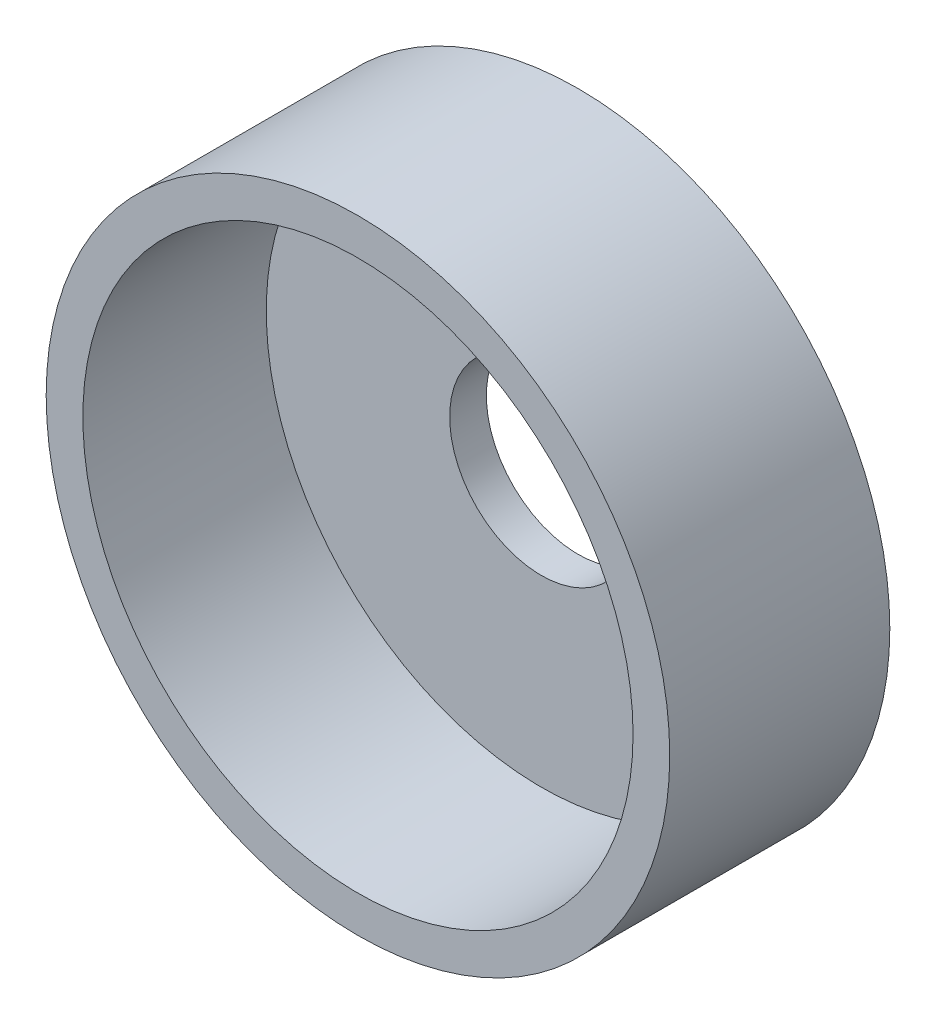
SolidWorks part; units mm, degrees
material "Q235A"
ref_plane "Front Plane" through (0, 0, 0) normal (0, 0, 1) x (1, 0, 0)
ref_plane "Top Plane" through (0, 0, 0) normal (0, 1, 0) x (1, 0, 0)
ref_plane "Right Plane" through (0, 0, 0) normal (1, 0, 0) x (0, 0, -1)
sketch "Sketch1" plane through (0, 0, 0) normal (0, 0, 1) x (1, 0, 0)
  circle A0 centre (0, 0) radius 8.5
  circle A1 centre (0, 0) radius 2.5
  dimension "D1" = 17
  dimension "D2" = 5
extrude "Boss-Extrude1" add sketch "Sketch1" along normal blind 6
sketch "Sketch2" plane through (0, 0, 6) normal (0, 0, 1) x (1, 0, 0)
  circle A0 centre (0, 0) radius 7.5
  circle A1 centre (0, 0) radius 8.5 construction
  dimension "D1" = 1
extrude "Cut-Extrude1" cut sketch "Sketch2" against normal blind 5
